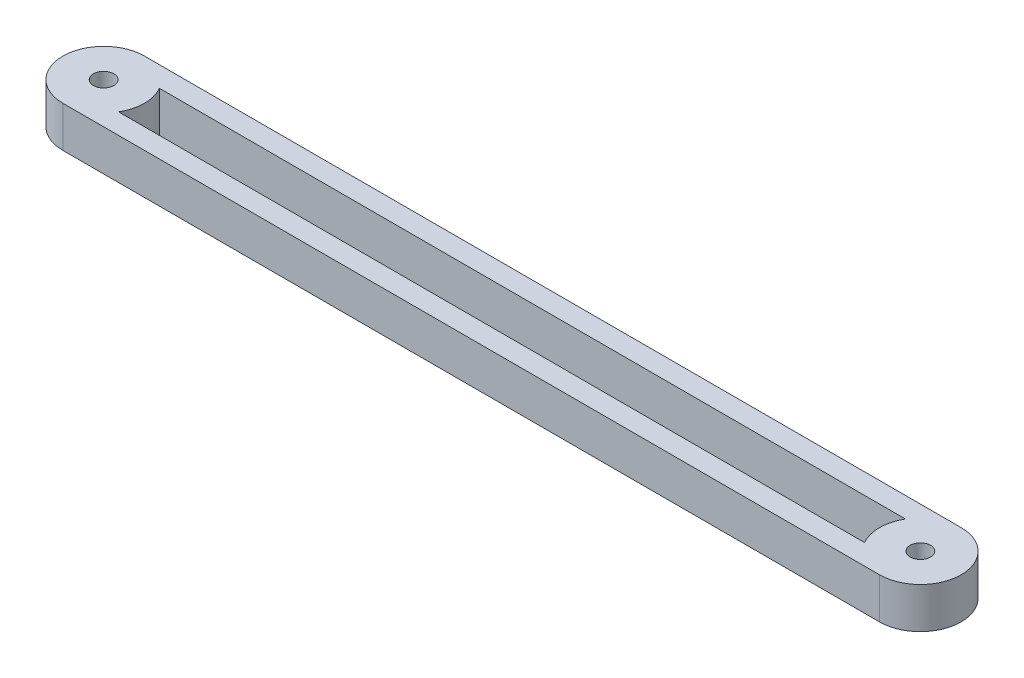
from build123d import *

# Parameters (mm, degrees)
SKETCH1_W           = 400
SKETCH1_H           = 40
BOSS_EXTRUDE1_DEPTH = 20
SKETCH2_W           = 380
SKETCH2_H           = 20
CUT_EXTRUDE1_DEPTH  = 202.990098767
SKETCH4_R           = 20
BOSS_EXTRUDE2_DEPTH = 20
SKETCH6_R           = 5
CUT_EXTRUDE2_DEPTH  = 222.810730128


with BuildPart() as part:
    # Sketch1 → Boss-Extrude1 (new body)
    with BuildSketch(Plane(origin=(0, 0, 0), x_dir=(1, 0, 0), z_dir=(0, 1, 0))):
        Rectangle(SKETCH1_W, SKETCH1_H)
    extrude(amount=BOSS_EXTRUDE1_DEPTH)

    # Sketch2 → Cut-Extrude1 (cut, through all)
    with BuildSketch(Plane(origin=(0, 20, 0), x_dir=(1, 0, 0), z_dir=(0, 1, 0))):
        Rectangle(SKETCH2_W, SKETCH2_H)
    extrude(amount=-CUT_EXTRUDE1_DEPTH, mode=Mode.SUBTRACT)

    # Sketch4 → Boss-Extrude2 (add)
    with BuildSketch(Plane(origin=(0, 20, 0), x_dir=(1, 0, 0), z_dir=(0, 1, 0))):
        with Locations((200, 0)):
            Circle(SKETCH4_R)
        with Locations((-200, 0)):
            Circle(SKETCH4_R)
    extrude(amount=-BOSS_EXTRUDE2_DEPTH)

    # Sketch6 → Cut-Extrude2 (cut, through all)
    with BuildSketch(Plane(origin=(0, 20, 0), x_dir=(1, 0, 0), z_dir=(0, 1, 0))):
        with Locations(Location((200, 0, 0), (0, 0, 270))):
            Circle(SKETCH6_R)
        with Locations(Location((-200, 0, 0), (0, 0, 90))):
            Circle(SKETCH6_R)
    extrude(amount=-CUT_EXTRUDE2_DEPTH, mode=Mode.SUBTRACT)


solid = part.part
